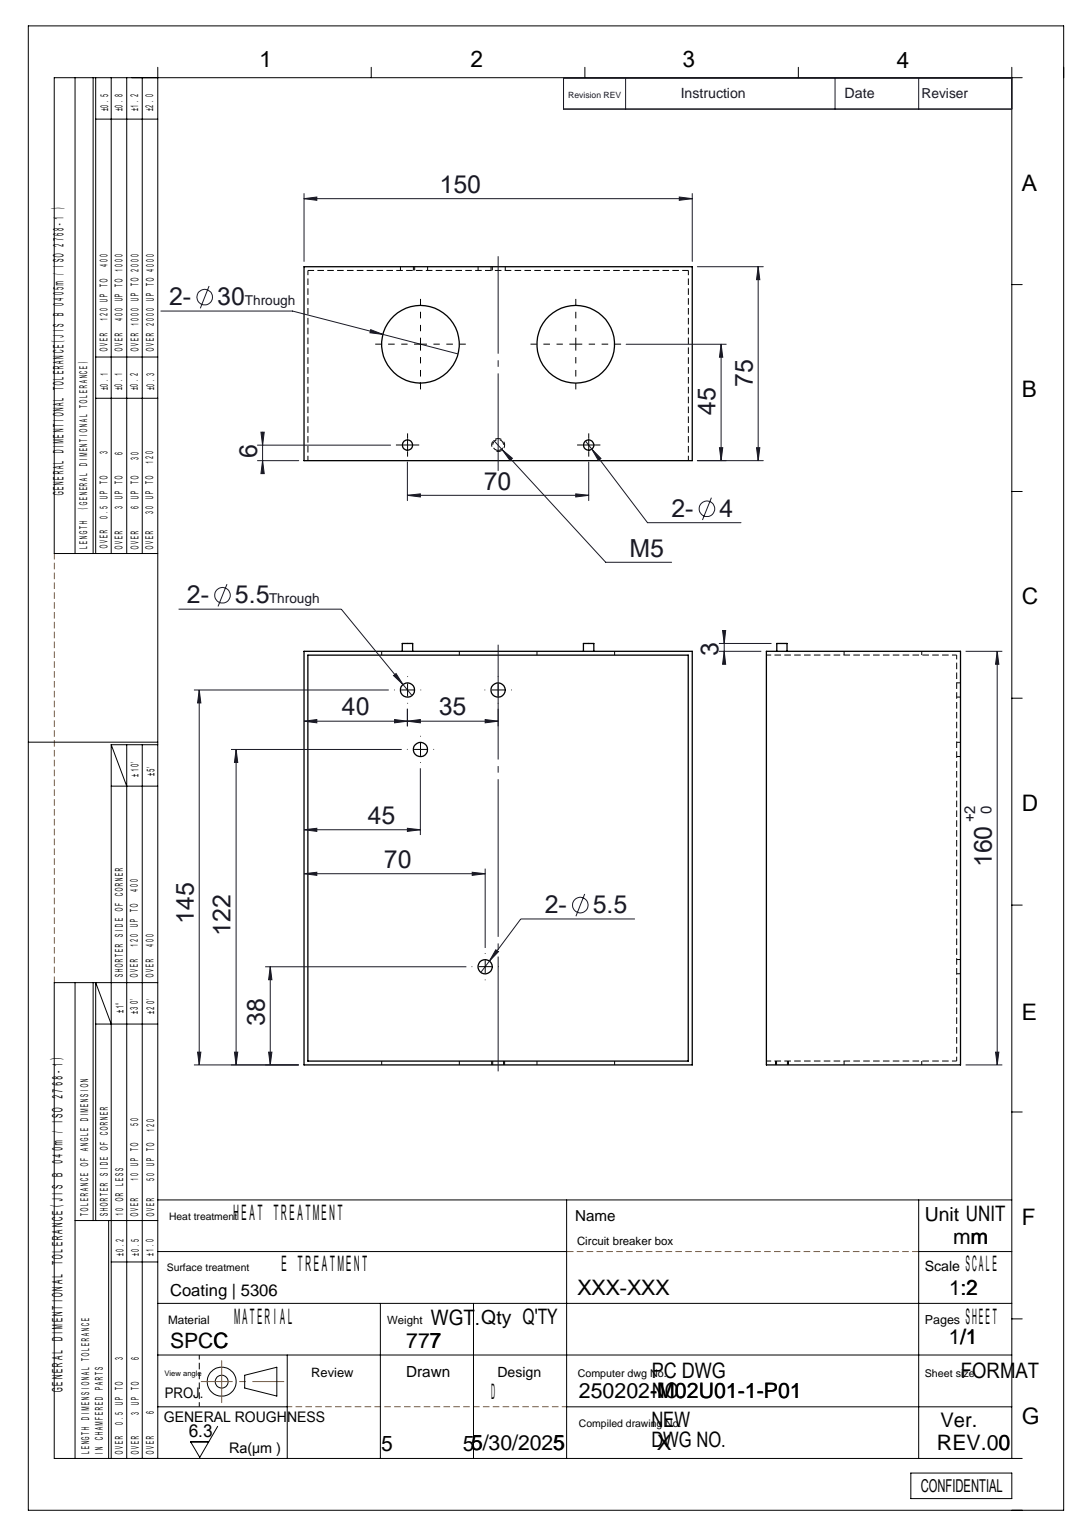
from build123d import *

# Parameters (mm, degrees)
SKETCH1_W                      = 150
SKETCH1_H                      = 160
BOSS_EXTRUDE1_DEPTH            = 37.5
SHELL1_T                       = -1.5
F_5_5_5_5_DIAMETER_HOLE2_D     = 5.5
SKETCH6_R                      = 15
CUT_EXTRUDE2_DEPTH             = 181.641218995
SKETCH8_R                      = 2
BOSS_EXTRUDE2_DEPTH            = 3
M5_TAPPED_HOLE1_D              = 4.2
M5_TAPPED_HOLE1_DEPTH          = 14
M5_TAPPED_HOLE1_TIP            = 1.2618073
F_5_5_5_5_DIAMETER_HOLE1_D     = 5.5
F_5_5_5_5_DIAMETER_HOLE1_DEPTH = 15
F_5_5_5_5_DIAMETER_HOLE1_TIP   = 1.652366702


with BuildPart() as part:
    # Sketch1 → Boss-Extrude1 (new, symmetric)
    with BuildSketch(Plane.XY):
        Rectangle(SKETCH1_W, SKETCH1_H)
    extrude(amount=BOSS_EXTRUDE1_DEPTH, both=True)

    # Shell1
    shell1_openings = [part.faces().sort_by_distance(p)[0] for p in [
        (0, 0, 37.5),
    ]]
    offset(amount=SHELL1_T, openings=shell1_openings, kind=Kind.INTERSECTION)

    # Ø5.5 (5.5) Diameter Hole2 (through all)
    with Locations(Plane.XY.offset(-36)):
        with Locations((-30, 42), (-5, -42)):
            Hole(F_5_5_5_5_DIAMETER_HOLE2_D / 2)

    # Sketch6 → Cut-Extrude2 (cut, through all)
    with BuildSketch(Plane(origin=(0, 80, 0), x_dir=(1, 0, 0), z_dir=(0, 1, 0))):
        with Locations(Location((-30, 7.5, 0), (0, 0, 270))):
            Circle(SKETCH6_R)
        with Locations(Location((30, 7.5, 0), (0, 0, 270))):
            Circle(SKETCH6_R)
    extrude(amount=-CUT_EXTRUDE2_DEPTH, mode=Mode.SUBTRACT)

    # Sketch8 → Boss-Extrude2 (add)
    with BuildSketch(Plane(origin=(0, 80, 0), x_dir=(1, 0, 0), z_dir=(0, 1, 0))):
        with Locations(Location((-35, -31.5, 0), (0, 0, 90))):
            Circle(SKETCH8_R)
        with Locations(Location((35, -31.5, 0), (0, 0, 90))):
            Circle(SKETCH8_R)
    extrude(amount=BOSS_EXTRUDE2_DEPTH)

    # M5 Tapped Hole1
    with Locations(Plane.XZ.offset(80)):
        with Locations((0, 31.5)):
            Hole(M5_TAPPED_HOLE1_D / 2, depth=M5_TAPPED_HOLE1_DEPTH)
            with Locations((0, 0, -(M5_TAPPED_HOLE1_DEPTH + M5_TAPPED_HOLE1_TIP / 2))):  # 118° drill point
                Cone(0, M5_TAPPED_HOLE1_D / 2, M5_TAPPED_HOLE1_TIP, mode=Mode.SUBTRACT)

    # Ø5.5 (5.5) Diameter Hole1
    with Locations(Plane.XY.offset(-36)):
        with Locations((0, 65), (-35, 65)):
            Hole(F_5_5_5_5_DIAMETER_HOLE1_D / 2, depth=F_5_5_5_5_DIAMETER_HOLE1_DEPTH)
            with Locations((0, 0, -(F_5_5_5_5_DIAMETER_HOLE1_DEPTH + F_5_5_5_5_DIAMETER_HOLE1_TIP / 2))):  # 118° drill point
                Cone(0, F_5_5_5_5_DIAMETER_HOLE1_D / 2, F_5_5_5_5_DIAMETER_HOLE1_TIP, mode=Mode.SUBTRACT)


solid = part.part
